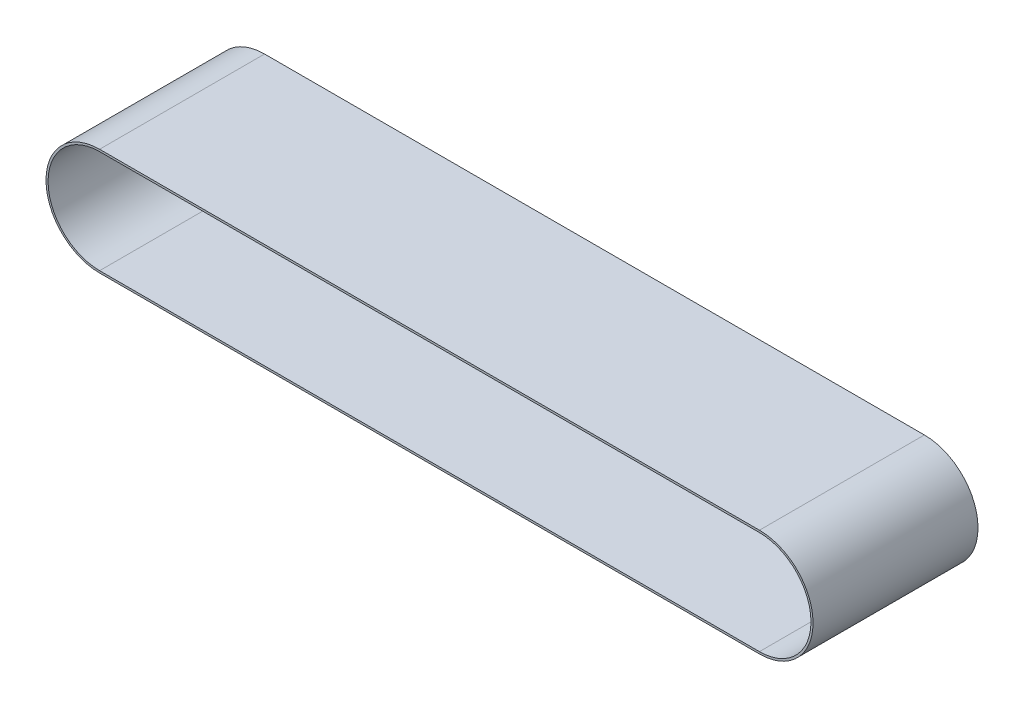
from build123d import *

# Parameters (mm, degrees)
BOSS_EXTRUDE1_DEPTH = 80


with BuildPart() as part:
    # Sketch1 → Boss-Extrude1 (new body)
    with BuildSketch(Plane.XY):
        with BuildLine():
            Line((320, -26), (0, -26))
            ThreePointArc((0, -26), (-26, 0), (0, 26))
            Line((0, 26), (320, 26))
            ThreePointArc((320, 26), (346, 0), (320, -26))
        make_face()
        with BuildLine():
            Line((0, 25), (320, 25))
            ThreePointArc((320, 25), (345, 0), (320, -25))
            Line((320, -25), (0, -25))
            ThreePointArc((0, -25), (-25, 0), (0, 25))
        make_face(mode=Mode.SUBTRACT)
    extrude(amount=BOSS_EXTRUDE1_DEPTH)


solid = part.part
